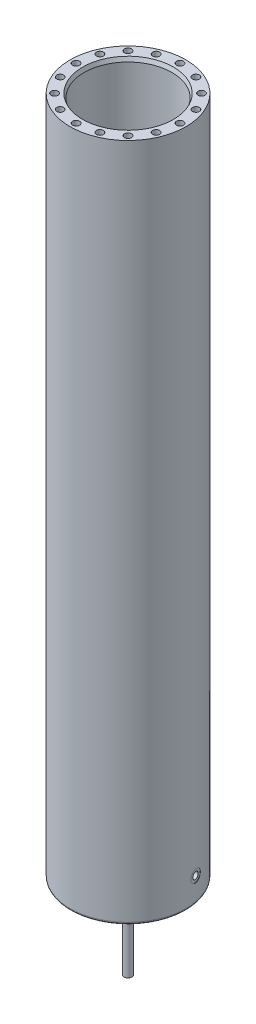
from build123d import *

# Parameters (mm, degrees)
M20_TAPPED_HOLE1_D                                   = 17.5
M20_TAPPED_HOLE1_DEPTH                               = 57.5
M20_TAPPED_HOLE1_TIP                                 = 5.257530416
HOLE_SIZE_PER_SOCKET_HEAD_CAP_SCREW_TYPE_D           = 12
HOLE_SIZE_PER_SOCKET_HEAD_CAP_SCREW_TYPE_DEPTH       = 50
HOLE_SIZE_PER_SOCKET_HEAD_CAP_SCREW_TYPE_CBORE_D     = 30
HOLE_SIZE_PER_SOCKET_HEAD_CAP_SCREW_TYPE_CBORE_DEPTH = 1
HOLE_SIZE_PER_SOCKET_HEAD_CAP_SCREW_TYPE_TIP         = 3.605163714
M18X1_5_TAPPED_HOLE1_D                               = 16.5
M18X1_5_TAPPED_HOLE1_DEPTH                           = 27.5
M18X1_5_TAPPED_HOLE1_TIP                             = 4.957100107
SKETCH7_R                                            = 25
BOSS_EXTRUDE1_DEPTH                                  = 10
SKETCH8_R                                            = 10
BOSS_EXTRUDE2_DEPTH                                  = 200


with BuildPart() as part:
    # Sketch1 → Revolve1 (revolve)
    with BuildSketch(Plane.XY, mode=Mode.PRIVATE) as revolve1_sk:
        with BuildLine():
            Line((0, 0), (-139, 0))
            ThreePointArc((-139, 0), (-143.242640687, 1.757359313), (-145, 6))
            Line((-145, 6), (-145, 1701))
            Line((-145, 1701), (-113.639702343, 1701))
            Line((-113.639702343, 1701), (-110, 1691))
            Line((-110, 1691), (-110, 50))
            ThreePointArc((-110, 50), (-108.535533906, 46.464466094), (-105, 45))
            Line((-105, 45), (0, 45))
            Line((0, 45), (0, 0))
        make_face()
    revolve(revolve1_sk.sketch.rotate(Axis((0, 0, 0), (0, 1, 0)), 270), axis=Axis((0, 0, 0), (0, 1, 0)))

    # M20 Tapped Hole1
    with Locations(Plane(origin=(0, 1701, 0), x_dir=(1, 0, 0), z_dir=(0, 1, 0))):
        with Locations((-130, 0), (-120.104339226, 49.748846207), (-91.923881554, 91.923881554), (-49.748846207, 120.104339226), (0, 130), (49.748846207, 120.104339226), (91.923881554, 91.923881554), (120.104339226, 49.748846207), (130, 0), (120.104339226, -49.748846207), (91.923881554, -91.923881554), (49.748846207, -120.104339226), (0, -130), (-49.748846207, -120.104339226), (-91.923881554, -91.923881554), (-120.104339226, -49.748846207)):
            Hole(M20_TAPPED_HOLE1_D / 2, depth=M20_TAPPED_HOLE1_DEPTH)
            with Locations((0, 0, -(M20_TAPPED_HOLE1_DEPTH + M20_TAPPED_HOLE1_TIP / 2))):  # 118° drill point
                Cone(0, M20_TAPPED_HOLE1_D / 2, M20_TAPPED_HOLE1_TIP, mode=Mode.SUBTRACT)

    # Hole size per socket head cap screw type1
    with Locations(Plane(origin=(142.3359416, 62, -27.66730433), x_dir=(0.190808995377, 0, 0.981627183448), z_dir=(0.981627183448, 0, -0.190808995377))):
        with Locations((0, 0)):
            CounterBoreHole(HOLE_SIZE_PER_SOCKET_HEAD_CAP_SCREW_TYPE_D / 2, HOLE_SIZE_PER_SOCKET_HEAD_CAP_SCREW_TYPE_CBORE_D / 2, HOLE_SIZE_PER_SOCKET_HEAD_CAP_SCREW_TYPE_CBORE_DEPTH, depth=HOLE_SIZE_PER_SOCKET_HEAD_CAP_SCREW_TYPE_DEPTH)
            with Locations((0, 0, -(HOLE_SIZE_PER_SOCKET_HEAD_CAP_SCREW_TYPE_DEPTH + HOLE_SIZE_PER_SOCKET_HEAD_CAP_SCREW_TYPE_TIP / 2))):  # 118° drill point
                Cone(0, HOLE_SIZE_PER_SOCKET_HEAD_CAP_SCREW_TYPE_D / 2, HOLE_SIZE_PER_SOCKET_HEAD_CAP_SCREW_TYPE_TIP, mode=Mode.SUBTRACT)

    # M18x1.5 Tapped Hole1
    with Locations(Plane(origin=(141.354314416, 0, -27.476495334), x_dir=(-0.1908089953765457, 0, -0.9816271834476639), z_dir=(0.9816271834476639, 0, -0.1908089953765457))):
        with Locations((0, 62)):
            Hole(M18X1_5_TAPPED_HOLE1_D / 2, depth=M18X1_5_TAPPED_HOLE1_DEPTH)
            with Locations((0, 0, -(M18X1_5_TAPPED_HOLE1_DEPTH + M18X1_5_TAPPED_HOLE1_TIP / 2))):  # 118° drill point
                Cone(0, M18X1_5_TAPPED_HOLE1_D / 2, M18X1_5_TAPPED_HOLE1_TIP, mode=Mode.SUBTRACT)


with BuildPart() as body_2:
    # Sketch7 → Boss-Extrude1 (new body)
    with BuildSketch(Plane.XZ):
        with Locations(Location((0, 0, 0), (0, 0, 270))):
            Circle(SKETCH7_R)
    extrude(amount=BOSS_EXTRUDE1_DEPTH)

    # Sketch8 → Boss-Extrude2 (add)
    with BuildSketch(Plane.XZ.offset(10)):
        with Locations(Location((0, 0, 0), (0, 0, 270))):
            Circle(SKETCH8_R)
    extrude(amount=BOSS_EXTRUDE2_DEPTH)


solid = Compound([part.part, body_2.part])
